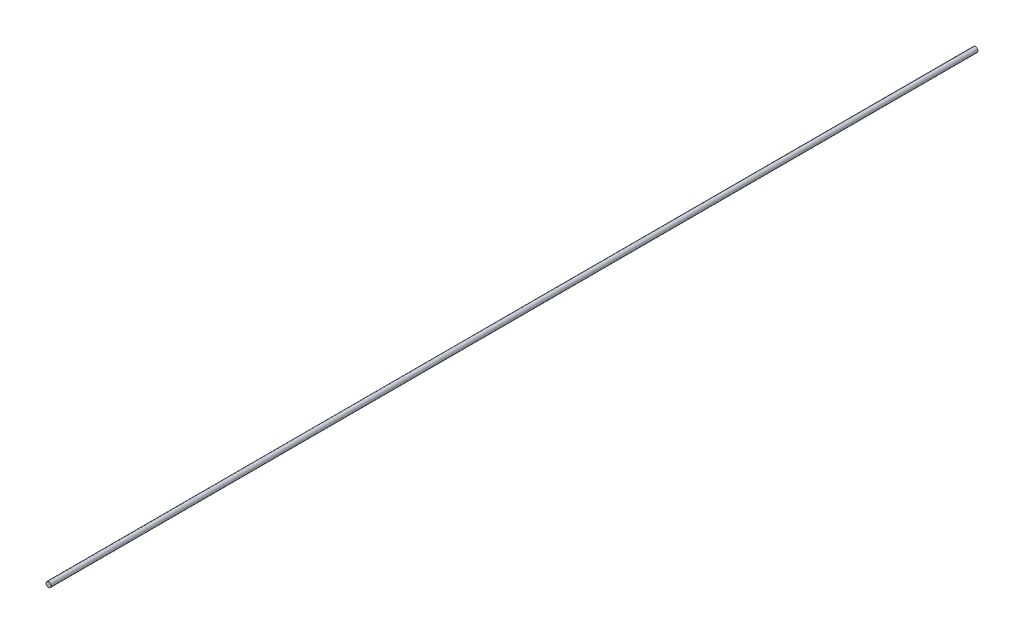
SolidWorks part; units mm, degrees
ref_plane "Front Plane" through (0, 0, 0) normal (0, 0, 1) x (1, 0, 0)
ref_plane "Top Plane" through (0, 0, 0) normal (0, 1, 0) x (1, 0, 0)
ref_plane "Right Plane" through (0, 0, 0) normal (1, 0, 0) x (0, 0, -1)
sketch "Sketch1" plane through (0, 0, 0) normal (0, 0, 1) x (1, 0, 0)
  circle A0 centre (0, 0) radius 15
  dimension "D1" = 30
extrude "Boss-Extrude1" add sketch "Sketch1" along normal blind 5500
